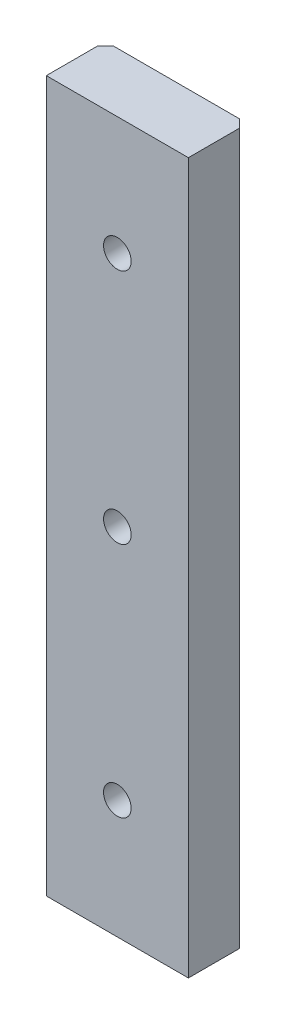
from build123d import *

# Parameters (mm, degrees)
SKETCH1_W           = 18
SKETCH1_H           = 7.5
BOSS_EXTRUDE1_DEPTH = 90
CHAMFER1_SIZE       = 1
SKETCH2_R           = 1.75
CUT_EXTRUDE1_DEPTH  = 91.759297044
SKETCH3_R           = 3
CUT_EXTRUDE2_DEPTH  = 4.5
LPATTERN1_COUNT     = 4
LPATTERN1_PITCH     = 30
LPATTERN2_COUNT     = 4
LPATTERN2_PITCH     = 30


with BuildPart() as part:
    # Sketch1 → Boss-Extrude1 (new body)
    with BuildSketch(Plane(origin=(0, 0, 0), x_dir=(1, 0, 0), z_dir=(0, 1, 0))):
        Rectangle(SKETCH1_W, SKETCH1_H)
    extrude(amount=BOSS_EXTRUDE1_DEPTH)

    # Chamfer1
    chamfer1_edges = [part.edges().sort_by_distance(p)[0] for p in [
        (-9, 45, -3.75),
        (9, 45, -3.75),
    ]]
    chamfer(chamfer1_edges, length=CHAMFER1_SIZE)

    # Sketch2 → Cut-Extrude1 (cut, through all)
    with BuildSketch(Plane(origin=(0, 0, -3.75), x_dir=(-1, 0, 0), z_dir=(0, 0, -1))):
        with Locations((0, 15)):
            Circle(SKETCH2_R)
    cut_extrude1 = extrude(amount=-CUT_EXTRUDE1_DEPTH, mode=Mode.SUBTRACT)

    # Sketch3 → Cut-Extrude2 (cut)
    with BuildSketch(Plane(origin=(0, 0, -3.75), x_dir=(-1, 0, 0), z_dir=(0, 0, -1))):
        with Locations((0, 15)):
            Circle(SKETCH3_R)
    cut_extrude2 = extrude(amount=-CUT_EXTRUDE2_DEPTH, mode=Mode.SUBTRACT)

    # LPattern1: Cut-Extrude2 ×4
    with Locations(*[(0, i * LPATTERN1_PITCH, 0) for i in range(1, LPATTERN1_COUNT)]):
        add(cut_extrude2, mode=Mode.SUBTRACT)

    # LPattern2: Cut-Extrude1 ×4
    with Locations(*[(0, i * LPATTERN2_PITCH, 0) for i in range(1, LPATTERN2_COUNT)]):
        add(cut_extrude1, mode=Mode.SUBTRACT)


solid = part.part
